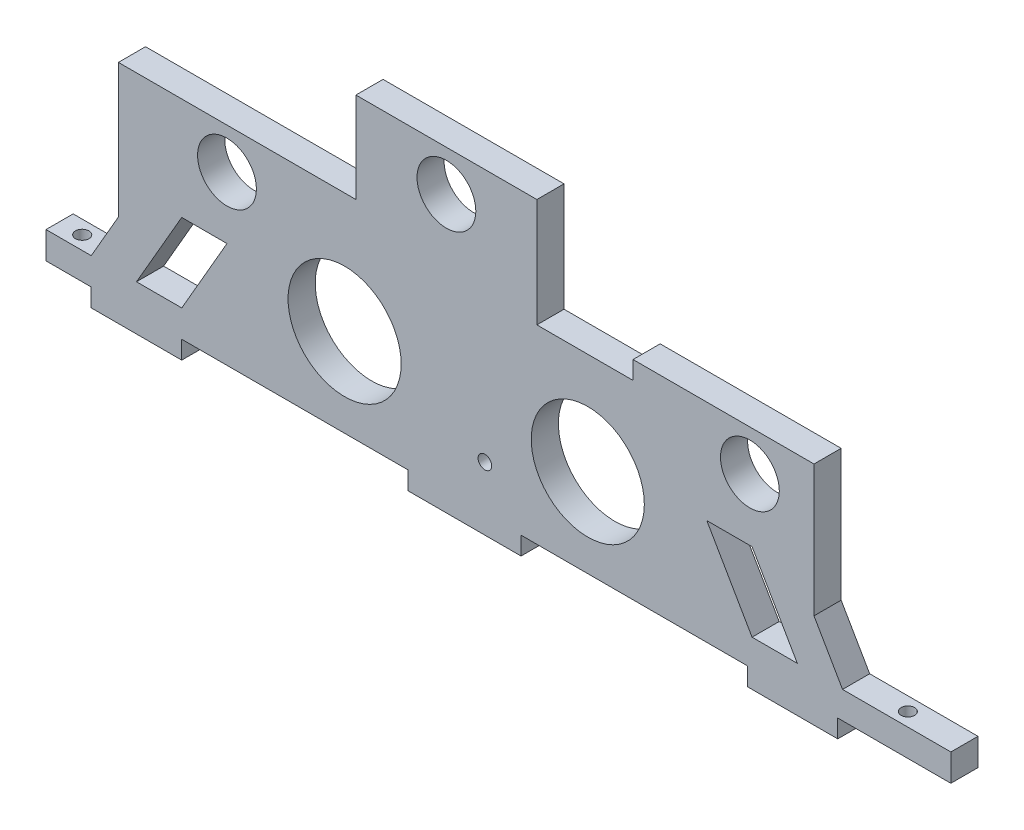
SolidWorks part; units mm, degrees
ref_plane "Front Plane" through (0, 0, 0) normal (0, 0, 1) x (1, 0, 0)
ref_plane "Top Plane" through (0, 0, 0) normal (0, 1, 0) x (1, 0, 0)
ref_plane "Right Plane" through (0, 0, 0) normal (1, 0, 0) x (0, 0, -1)
other "Configuration Table"
sketch "Sketch1" plane through (0, 0, 0) normal (0, 0, 1) x (1, 0, 0)
  line L1 (-100, 22.5) -> (100, 22.5)
  line L2 (-100, 22.5) -> (-100, -22.5)
  line L3 (-100, -22.5) -> (100, -22.5)
  line L4 (100, 22.5) -> (100, -22.5)
  line L5 (0, -22.5) -> (0, 22.5) construction
  line L6 (-100, 0) -> (100, 0) construction
  point P0 (0, 0)
  dimension "D1" = 200
  dimension "D2" = 45
extrude "Boss-Extrude1" add sketch "Sketch1" along normal blind 6
sketch "Sketch2" plane through (0, 0, 6) normal (0, 0, 1) x (1, 0, 0)
  line L0 (-90, -19.5) -> (-90, -22.5)
  line L1 (-100, -22.5) -> (100, -22.5) construction
  line L2 (-100, 22.5) -> (-100, -22.5) construction
  line L3 (-90, -22.5) -> (-70, -22.5) construction
  line L4 (-70, -22.5) -> (-70, -19.5)
  line L5 (-70, -19.5) -> (-20, -19.5)
  line L6 (-20, -19.5) -> (-20, -22.5)
  line L7 (-20, -22.5) -> (5, -22.5) construction
  line L8 (5, -22.5) -> (5, -19.5)
  line L9 (5, -19.5) -> (55, -19.5)
  line L10 (55, -19.5) -> (55, -22.5)
  line L11 (55, -22.5) -> (75, -22.5) construction
  line L12 (75, -22.5) -> (75, -19.5)
  line L13 (75, -19.5) -> (100, -19.5)
  line L14 (100, -22.5) -> (100, 22.5) construction
  line L15 (5, -22.5) -> (55, -22.5)
  line L16 (-90, -19.5) -> (-100, -19.5)
  line L17 (-100, -19.5) -> (-100, -22.5)
  line L18 (-100, -22.5) -> (-90, -22.5)
  line L19 (-70, -22.5) -> (-20, -22.5)
  line L20 (75, -22.5) -> (100, -22.5)
  line L21 (100, -22.5) -> (100, -19.5)
  dimension "D1" = 3
  dimension "D2" = 10
  dimension "D3" = 20
  dimension "D4" = 50
  dimension "D5" = 25
  dimension "D6" = 50
  dimension "D7" = 20
extrude "Cut-Extrude1" cut sketch "Sketch2" against normal up to next
sketch "Sketch3" plane through (0, 0, 6) normal (0, 0, 1) x (1, 0, 0)
  line L0 (-11.5, 46.0715) -> (-11.5, -46.2113) construction
  line L1 (-100, 22.5) -> (-100, -19.5) construction
  line L2 (-11.5, 17.5) -> (42.7759, 17.5) construction
  line L3 (-20, -22.5) -> (5, -22.5) construction
  line L4 (-31.5, 42.5) -> (-31.5, 22.5)
  line L5 (-5, 37.5) -> (-2, 37.5)
  line L6 (-18, 37.5) -> (-21, 37.5)
  line L7 (-2, 37.5) -> (-2, 42.5)
  line L8 (-21, 37.5) -> (-21, 42.5)
  line L9 (-21, 42.5) -> (-31.5, 42.5)
  line L10 (-2, 42.5) -> (8.5, 42.5)
  line L11 (100, 22.5) -> (-100, 22.5) construction
  line L12 (8.5, 42.5) -> (8.5, 22.5)
  line L13 (8.5, 22.5) -> (-31.5, 22.5)
  arc A1 (-18, 37.5) -> (-5, 37.5) centre (-11.5, 37.5) ccw
  dimension "D3" = 3
  dimension "D4" = 13
  dimension "D1" = 88.5
  dimension "D2" = 40
  dimension "D5" = 20
  dimension "D6" = 3
  dimension "D7" = 5
  dimension "D8" = 5
  dimension "D9" = 10.5
  dimension "D10" = 10.5
extrude "Boss-Extrude2" add sketch "Sketch3" against normal up to surface (6 mm away) up to face at (-5.625, -15.375, 0)
sketch "Sketch4" plane through (0, 0, 6) normal (0, 0, 1) x (1, 0, 0)
  line L0 (-11.5, 37.5) -> (-11.5, -30.1891) construction
  line L1 (-11.5, 17.5) -> (29.3686, 17.5) construction
  line L2 (-20, -22.5) -> (5, -22.5) construction
  line L4 (-90, -22.5) -> (-70, -22.5) construction
  line L5 (55, -22.5) -> (75, -22.5) construction
  line L7 (-53.5, 17.5) -> (-50.5, 17.5)
  line L8 (-66.5, 17.5) -> (-69.5, 17.5)
  line L9 (-50.5, 17.5) -> (-50.5, 22.5)
  line L10 (-69.5, 17.5) -> (-69.5, 22.5)
  line L11 (-31.5, 22.5) -> (-100, 22.5) construction
  line L13 (53, 17.5) -> (56, 17.5)
  line L14 (56, 17.5) -> (56, 22.5)
  line L15 (100, 22.5) -> (8.5, 22.5) construction
  line L16 (40, 17.5) -> (37, 17.5)
  line L17 (37, 17.5) -> (37, 22.5)
  line L18 (37, 22.5) -> (56, 22.5)
  line L19 (-69.5, 22.5) -> (-50.5, 22.5)
  arc A0 (-66.5, 17.5) -> (-53.5, 17.5) centre (-60, 17.5) ccw
  arc A1 (40, 17.5) -> (53, 17.5) centre (46.5, 17.5) ccw
  dimension "D2" = 13
  dimension "D5" = 13
  dimension "D1" = 40
  dimension "D3" = 48.5
  dimension "D4" = 40
  dimension "D6" = 40
  dimension "D7" = 3
  dimension "D8" = 3
  dimension "D9" = 5
  dimension "D10" = 3
  dimension "D11" = 3
  dimension "D12" = 58
extrude "Cut-Extrude2" cut sketch "Sketch4" against normal up to surface (6 mm away) up to face at (-7.8846, 4.3269, 0)
sketch "Sketch5" plane through (0, 22.5, 0) normal (0, 1, 0) x (1, 0, 0)
  line L0 (-69.5, 0) -> (-69.5, -6) construction
  line L1 (-69.5, -6) -> (-100, -6) construction
  line L2 (-80, -6) -> (-80, 0) construction
  line L3 (-69.5, 0) -> (-100, 0) construction
  line L4 (-50.5, -3) -> (-40, -3) construction
  line L5 (-69.5, -3) -> (-78.7031, -3) construction
  line L6 (-69.5, 0) -> (-69.5, -6) construction
  line L7 (-75, -3) -> (-75, -0.5069) construction
  line L9 (-50.5, 0) -> (-50.5, -6) construction
  line L10 (-45, -3) -> (-45, -0.762) construction
  line L11 (37, -3) -> (26.5, -3) construction
  line L13 (37, 0) -> (37, -6) construction
  line L14 (56, -3) -> (66.5, -3) construction
  line L15 (56, 0) -> (56, -6) construction
  line L16 (31.5, -3) -> (31.5, -0.5069) construction
  line L18 (61.5, -3) -> (61.5, -0.5069) construction
  dimension "D1" = 10.5
  dimension "D2" = 5
  dimension "D3" = 10.5
  dimension "D4" = 5
  dimension "D5" = 10.5
  dimension "D6" = 10.5
  dimension "D7" = 5
  dimension "D8" = 5
sketch "Sketch8" plane through (0, 42.5, 0) normal (0, 1, 0) x (1, 0, 0)
  line L0 (-21, -3) -> (-31.5, -3) construction
  line L1 (-21, 0) -> (-21, -6) construction
  line L2 (-26.5, -3) -> (-26.5, -0.7035) construction
  line L3 (-21, 0) -> (-21, -6) construction
  line L4 (-2, -3) -> (8.5, -3) construction
  line L5 (-2, 0) -> (-2, -6) construction
  line L6 (3.5, -3) -> (3.5, -0.458) construction
  line L7 (-2, 0) -> (-2, -6) construction
  dimension "D1" = 10.5
  dimension "D2" = 5.5
  dimension "D3" = 10.5
  dimension "D4" = 5.5
sketch "Sketch11" plane through (0, 0, 6) normal (0, 0, 1) x (1, 0, 0)
  line L0 (-100, -19.5) -> (-100, -13.5) construction
  line L1 (-100, 22.5) -> (-100, -19.5) construction
  line L2 (-100, -13.5) -> (-90, -13.5)
  line L3 (-90, -13.5) -> (-84, -3.1077)
  line L4 (-84, -3.1077) -> (-84, 22.5)
  line L5 (-69.5, 22.5) -> (-100, 22.5) construction
  line L6 (-84, 22.5) -> (-100, 22.5)
  line L7 (-100, 22.5) -> (-100, -13.5)
  line L8 (100, -19.5) -> (100, -13.5) construction
  line L9 (100, -19.5) -> (100, 22.5) construction
  line L10 (100, -13.5) -> (76.06, -13.5)
  line L11 (76.06, -13.5) -> (69.75, -2.5708)
  line L12 (69.75, -2.5708) -> (69.75, 22.5)
  line L13 (100, 22.5) -> (56, 22.5) construction
  line L14 (69.75, 22.5) -> (100, 22.5)
  line L15 (100, 22.5) -> (100, -13.5)
  dimension "D1" = 6
  dimension "D2" = 10
  dimension "D3" = 12
  dimension "D4" = 120
  dimension "D5" = 6
  dimension "D6" = 23.94
  dimension "D7" = 12.62
  dimension "D8" = 120
extrude "Cut-Extrude3" cut sketch "Sketch11" against normal up to surface (6 mm away) up to face at (-7.5263, 8.6711, 0)
sketch "Sketch12" plane through (0, -13.5, 0) normal (0, 1, 0) x (1, 0, 0)
  line L0 (-100, -3) -> (-90.9673, -3) construction
  line L1 (-100, 0) -> (-100, -6) construction
  line L2 (-95, -3) -> (-95, -0.4306) construction
  line L4 (100, -3) -> (79.3364, -3) construction
  line L5 (100, 0) -> (100, -6) construction
  line L6 (87.5, -3) -> (87.5, -0.4306) construction
  dimension "D1" = 5
  dimension "D2" = 12.5
sketch "Sketch15" plane through (0, 0, 6) normal (0, 0, 1) x (1, 0, 0)
  line L0 (-90, -13.5) -> (-40.2542, -13.5) construction
  line L1 (-80, -13.5) -> (-70, 3.8205)
  line L2 (-90, -13.5) -> (-84, -3.1077) construction
  line L3 (-70, 3.8205) -> (-60, 3.8205)
  line L4 (-60, 3.8205) -> (-69.9883, -13.5)
  line L5 (-80, -13.5) -> (-69.9883, -13.5)
  line L6 (-3.8043, -13.5) -> (76.06, -13.5) construction
  line L7 (66.06, -13.5) -> (56.06, 3.8205)
  line L8 (69.75, -2.5708) -> (76.06, -13.5) construction
  line L9 (56.06, 3.8205) -> (46.06, 3.8205)
  line L10 (46.06, 3.8205) -> (56.06, -13.5)
  line L11 (56.06, -13.5) -> (66.06, -13.5)
  line L12 (-20, -19.5) -> (-70, -19.5) construction
  line L15 (-84, -3.1077) -> (-84, 22.5) construction
  line L16 (69.75, 22.5) -> (69.75, -2.5708) construction
  circle A0 centre (-34, 0) radius 12.5
  circle A1 centre (19.75, 0) radius 12.5
  dimension "D1" = 20
  dimension "D7" = 25
  dimension "D8" = 25
  dimension "D2" = 10
  dimension "D3" = 10
  dimension "D4" = 20
  dimension "D5" = 10
  dimension "D6" = 10
  dimension "D9" = 19.5
  dimension "D10" = 50
  dimension "D11" = 50
extrude "Cut-Extrude4" cut sketch "Sketch15" against normal up to surface (6 mm away) up to face at (-7.4645, 6.1323, 0)
sketch "Sketch16" plane through (0, 0, 6) normal (0, 0, 1) x (1, 0, 0)
  line L0 (-21.5112, -10) -> (6.5112, -10) construction
  line L1 (-20, -22.5) -> (5, -22.5) construction
  line L2 (-7.5, -10) -> (-7.5, -19.2249) construction
  line L3 (-100, -13.5) -> (-100, -19.5) construction
  dimension "D1" = 12.5
  dimension "D2" = 92.5
sketch "Sketch19" plane through (0, 0, 6) normal (0, 0, 1) x (1, 0, 0)
  line L0 (-84, 22.5) -> (-84, 26.5)
  line L1 (-84, 26.5) -> (-31.5, 26.5)
  line L2 (-31.5, 42.5) -> (-31.5, 22.5) construction
  line L3 (-31.5, 26.5) -> (-31.5, 22.5)
  line L4 (-31.5, 22.5) -> (-50.5, 22.5)
  line L5 (-50.5, 22.5) -> (-50.5, 17.5)
  line L6 (-50.5, 17.5) -> (-53.5, 17.5)
  line L7 (-66.5, 17.5) -> (-69.5, 17.5)
  line L8 (-69.5, 17.5) -> (-69.5, 22.5)
  line L9 (-69.5, 22.5) -> (-84, 22.5)
  line L10 (-31.5, 42.5) -> (-31.5, 46.5)
  line L11 (-31.5, 46.5) -> (8.5, 46.5)
  line L12 (8.5, 46.5) -> (8.5, 42.5)
  line L13 (8.5, 42.5) -> (-2, 42.5)
  line L14 (-2, 42.5) -> (-2, 37.5)
  line L15 (-2, 37.5) -> (-5, 37.5)
  line L16 (-18, 37.5) -> (-21, 37.5)
  line L17 (-21, 37.5) -> (-21, 42.5)
  line L18 (-21, 42.5) -> (-31.5, 42.5)
  line L19 (29.75, 22.5) -> (29.75, 26.5)
  line L20 (37, 22.5) -> (8.5, 22.5) construction
  line L21 (29.75, 26.5) -> (69.75, 26.5)
  line L22 (69.75, 26.5) -> (69.75, 22.5)
  line L23 (69.75, 22.5) -> (56, 22.5)
  line L24 (56, 22.5) -> (56, 17.5)
  line L25 (56, 17.5) -> (53, 17.5)
  line L26 (40, 17.5) -> (37, 17.5)
  line L27 (37, 17.5) -> (37, 22.5)
  line L28 (37, 22.5) -> (29.75, 22.5)
  arc A0 (-66.5, 17.5) -> (-53.5, 17.5) centre (-60, 17.5) ccw construction
  arc A1 (-66.5, 17.5) -> (-53.5, 17.5) centre (-60, 17.5) ccw
  circle A2 centre (-60, 17.5) radius 6.5
  arc A3 (-18, 37.5) -> (-5, 37.5) centre (-11.5, 37.5) ccw construction
  arc A4 (-18, 37.5) -> (-5, 37.5) centre (-11.5, 37.5) ccw construction
  circle A5 centre (-11.5, 37.5) radius 6.5
  arc A6 (40, 17.5) -> (53, 17.5) centre (46.5, 17.5) ccw construction
  arc A7 (40, 17.5) -> (53, 17.5) centre (46.5, 17.5) ccw construction
  circle A8 centre (46.5, 17.5) radius 6.5
  dimension "D1" = 4
  dimension "D2" = 4
  dimension "D3" = 4
  dimension "D4" = 40
extrude "Boss-Extrude3" add sketch "Sketch19" against normal blind 6 contours A2 L6 L5 L4 L3 L1 L0 L9 L8 L7 | A5 L15 L14 L13 L12 L11 L10 L18 L17 L16 | A8 L25 L24 L23 L22 L21 L19 L28 L27 L26
sketch "Sketch20" plane through (0, 0, 0) normal (0, 0, -1) x (-1, 0, 0)
  line L0 (-8.5, 46.5) -> (-8.5, 22.5) construction
  line L1 (-5, -19.5) -> (-55, -19.5) construction
  circle A0 centre (3, -9.5) radius 1.5
  dimension "D1" = 3
  dimension "D2" = 11.5
  dimension "D3" = 10
extrude "Cut-Extrude5" cut sketch "Sketch20" against normal through all
sketch "Sketch21" plane through (0, -13.5, 0) normal (0, 1, 0) x (1, 0, 0)
  line L0 (-100, -3) -> (123.6249, -3) construction
  line L1 (-100, 0) -> (-100, -6) construction
  line L2 (100, 0) -> (100, -6) construction
  circle A0 centre (87.5, -3) radius 1.5
  circle A1 centre (-95, -3) radius 1.5
  dimension "D1" = 3
  dimension "D3" = 3
  dimension "D2" = 12.5
  dimension "D4" = 5
extrude "Cut-Extrude6" cut sketch "Sketch21" against normal through all
sketch "Sketch22" plane through (0, 0, 0) normal (1, 0, 0) x (0, 0, -1)
  line L0 (0, -19.5) -> (5, -19.5)
  line L1 (5, -19.5) -> (5, -16.5)
  line L2 (5, -16.5) -> (2.5, -16.5)
  line L3 (2.5, -16.5) -> (0, -15)
  line L4 (0, -19.5) -> (0, -13.5) construction
  line L5 (0, -15) -> (0, -19.5)
  dimension "D1" = 3
  dimension "D2" = 1.5
  dimension "D3" = 5
  dimension "D4" = 2.5
sketch "Sketch23" plane through (0, 0, 0) normal (1, 0, 0) x (0, 0, -1)
  line L0 (-3, 46.5) -> (-3, -22.5) construction
  line L1 (0, 46.5) -> (-6, 46.5) construction
  line L2 (0, -22.5) -> (-6, -22.5) construction
ref_plane "Plane1" through (0, 0, 3) normal (0, 0, -1) x (-1, 0, 0)
sketch "Sketch24" plane through (0, -22.5, 0) normal (0, -1, 0) x (1, 0, 0)
  line L0 (-70, 6) -> (-90, 6) construction
  line L1 (-90, 6) -> (-90, 0) construction
  line L2 (-90, 0) -> (-70, 0) construction
  line L3 (-70, 0) -> (-70, 6) construction
  line L4 (-20, 0) -> (5, 0) construction
  line L5 (5, 0) -> (5, 6) construction
  line L6 (5, 6) -> (-20, 6) construction
  line L7 (-20, 6) -> (-20, 0) construction
  line L8 (75, 6) -> (55, 6) construction
  line L9 (55, 6) -> (55, 0) construction
  line L10 (55, 0) -> (75, 0) construction
  line L11 (75, 0) -> (75, 6) construction
  line L12 (-70, 6) -> (-90, 6)
  line L13 (-90, 6) -> (-90, 0)
  line L14 (-90, 0) -> (-70, 0)
  line L15 (-70, 0) -> (-70, 6)
  line L16 (-20, 0) -> (5, 0)
  line L17 (5, 0) -> (5, 6)
  line L18 (5, 6) -> (-20, 6)
  line L19 (-20, 6) -> (-20, 0)
  line L20 (75, 6) -> (55, 6)
  line L21 (55, 6) -> (55, 0)
  line L22 (55, 0) -> (75, 0)
  line L23 (75, 0) -> (75, 6)
extrude "Boss-Extrude4" add sketch "Sketch24" along normal blind 1
sketch "Sketch25" plane through (0, 0, 6) normal (0, 0, 1) x (1, 0, 0)
  circle A0 centre (46.5, 17.5) radius 6.5 construction
  circle A1 centre (-60, 17.5) radius 6.5 construction
  circle A2 centre (46.5, 17.5) radius 6.5
  circle A3 centre (-60, 17.5) radius 6.5
extrude "Boss-Extrude5" add sketch "Sketch25" against normal up to surface (6 mm away) up to face at (-4.5, -9.5, 0)
sketch "Sketch26" plane through (0, 0, 6) normal (0, 0, 1) x (1, 0, 0)
  line L0 (29.75, 26.5) -> (69.75, 26.5) construction
  line L1 (69.75, 26.5) -> (69.75, -2.5708) construction
  line L2 (-84, -3.1077) -> (-84, 26.5) construction
  line L3 (-84, 26.5) -> (-31.5, 26.5) construction
  circle A0 centre (55.58, 17.5) radius 6.5
  circle A1 centre (-60, 17.5) radius 6.5
  dimension "D1" = 9
  dimension "D2" = 13
  dimension "D4" = 13
  dimension "D3" = 14.17
  dimension "D5" = 24
  dimension "D6" = 9
extrude "Cut-Extrude7" cut sketch "Sketch26" against normal through all
